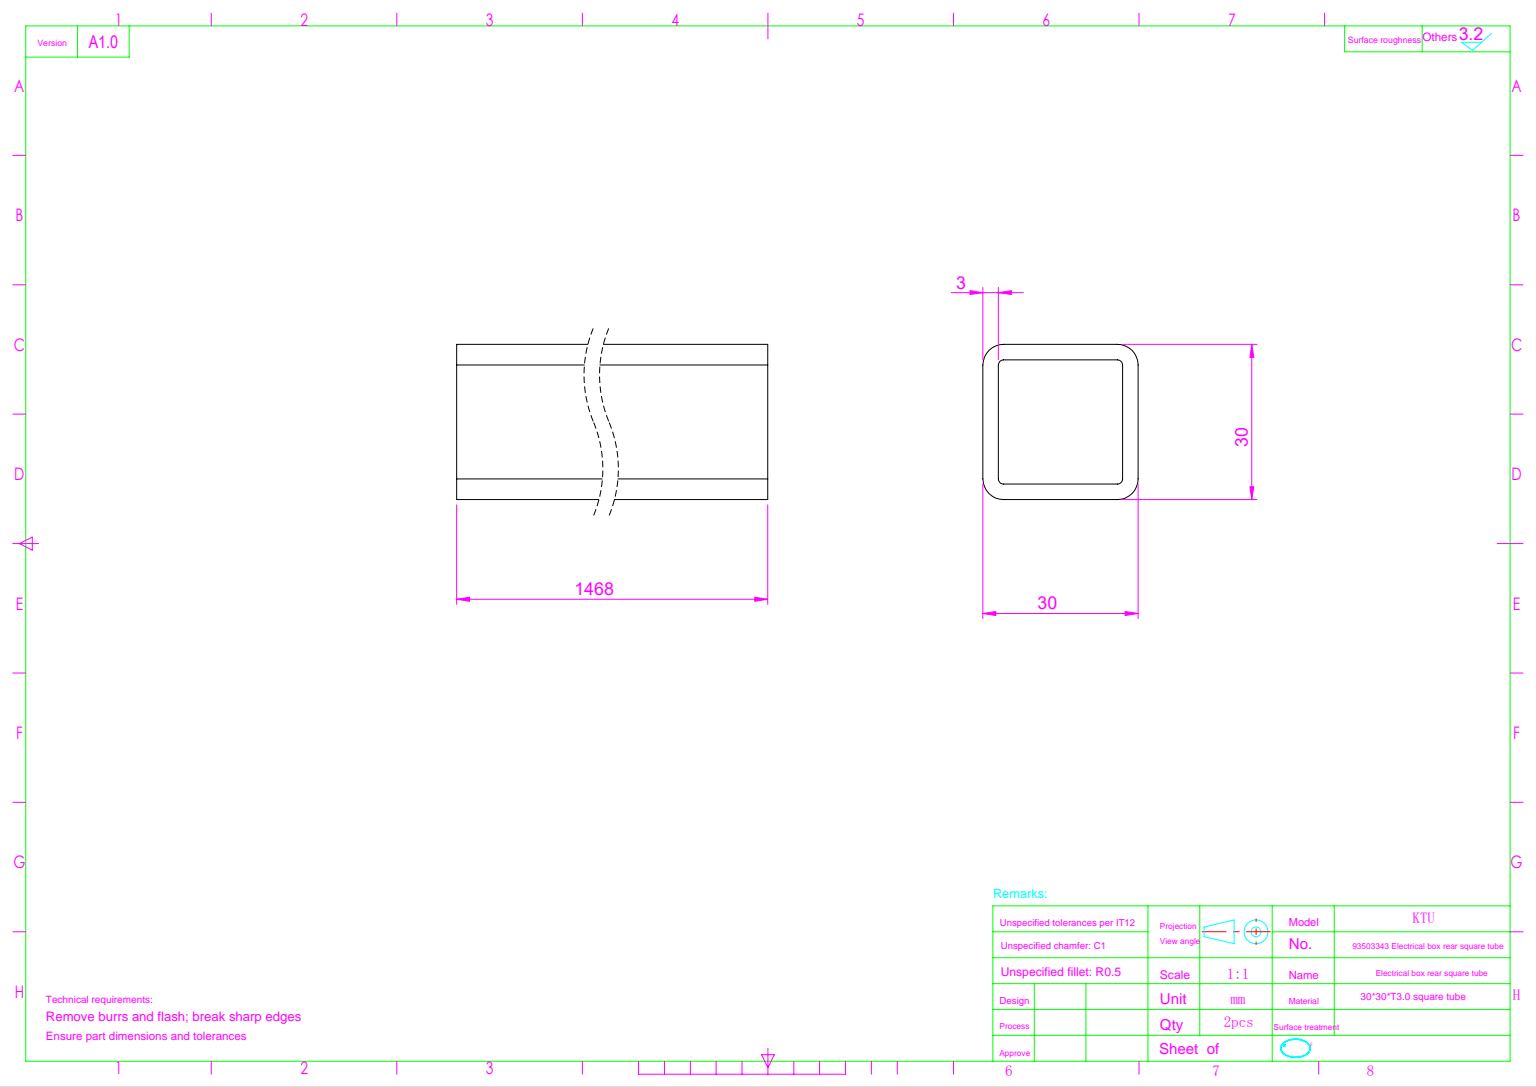
from build123d import *

# Parameters (mm, degrees)
EXTRUDE_1_DEPTH = 734


with BuildPart() as part:
    # 草图2 → 拉伸-薄壁1 (new, symmetric)
    with BuildSketch(Plane.XY):
        with BuildLine():
            Line((-11, 15), (11, 15))
            ThreePointArc((11, 15), (13.828427125, 13.828427125), (15, 11))
            Line((15, 11), (15, -11))
            ThreePointArc((15, -11), (13.828427125, -13.828427125), (11, -15))
            Line((11, -15), (-11, -15))
            ThreePointArc((-11, -15), (-13.828427125, -13.828427125), (-15, -11))
            Line((-15, -11), (-15, 11))
            ThreePointArc((-15, 11), (-13.828427125, 13.828427125), (-11, 15))
        make_face()
        with BuildLine():
            Line((-11, 12), (11, 12))
            ThreePointArc((11, 12), (11.707106781, 11.707106781), (12, 11))
            Line((12, 11), (12, -11))
            ThreePointArc((12, -11), (11.707106781, -11.707106781), (11, -12))
            Line((11, -12), (-11, -12))
            ThreePointArc((-11, -12), (-11.707106781, -11.707106781), (-12, -11))
            Line((-12, -11), (-12, 11))
            ThreePointArc((-12, 11), (-11.707106781, 11.707106781), (-11, 12))
        make_face(mode=Mode.SUBTRACT)
    extrude(amount=EXTRUDE_1_DEPTH, both=True)


solid = part.part
